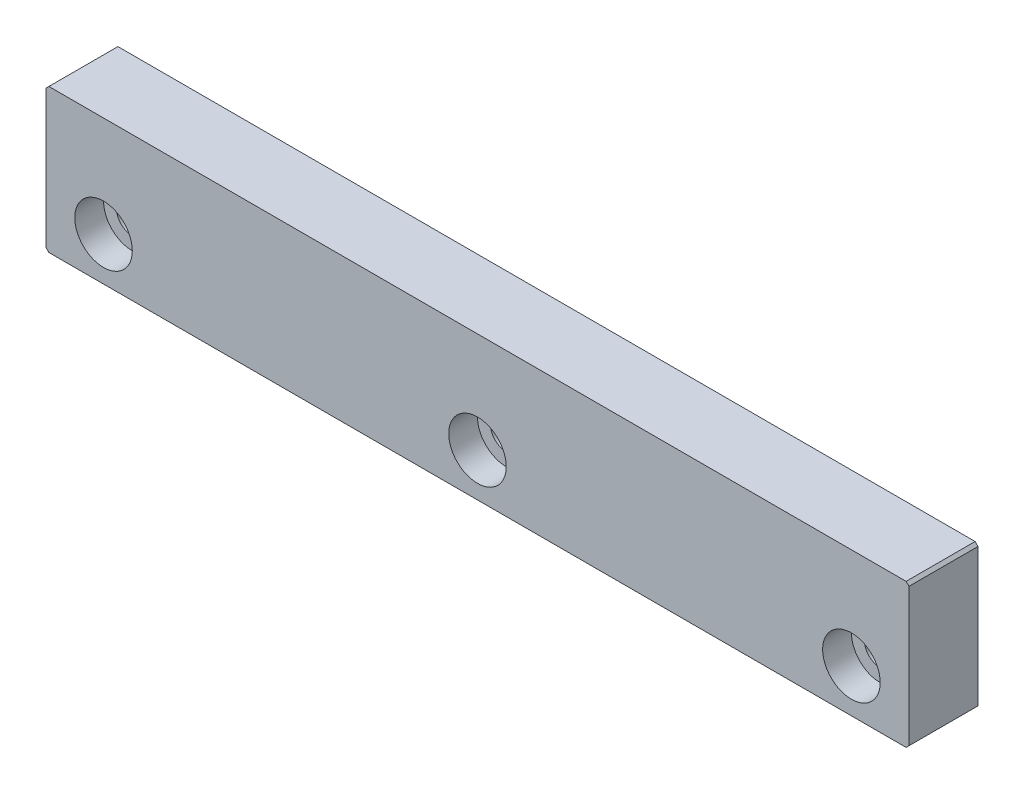
from build123d import *

# Parameters (mm, degrees)
SKETCH1_W                                           = 150
SKETCH1_H                                           = 25
BOSS_EXTRUDE1_DEPTH                                 = 12
CBORE_FOR_M5_HEX_SOCKET_HEAD_CAP_SCREW1_D           = 5.5
CBORE_FOR_M5_HEX_SOCKET_HEAD_CAP_SCREW1_CBORE_D     = 10
CBORE_FOR_M5_HEX_SOCKET_HEAD_CAP_SCREW1_CBORE_DEPTH = 5
CHAMFER1_SIZE                                       = 0.5


with BuildPart() as part:
    # Sketch1 → Boss-Extrude1 (new body)
    with BuildSketch(Plane.XY):
        Rectangle(SKETCH1_W, SKETCH1_H)
    extrude(amount=BOSS_EXTRUDE1_DEPTH)

    # CBORE for M5 Hex Socket Head Cap Screw1 (through all)
    with Locations(Plane.XY.offset(12)):
        with Locations((0, -5), (-65, -5), (65, -5)):
            CounterBoreHole(CBORE_FOR_M5_HEX_SOCKET_HEAD_CAP_SCREW1_D / 2, CBORE_FOR_M5_HEX_SOCKET_HEAD_CAP_SCREW1_CBORE_D / 2, CBORE_FOR_M5_HEX_SOCKET_HEAD_CAP_SCREW1_CBORE_DEPTH)

    # Chamfer1
    chamfer1_edges = [part.edges().sort_by_distance(p)[0] for p in [
        (75, -12.5, 6),
        (-75, -12.5, 6),
        (-75, 12.5, 6),
        (75, 12.5, 6),
    ]]
    chamfer(chamfer1_edges, length=CHAMFER1_SIZE)


solid = part.part
